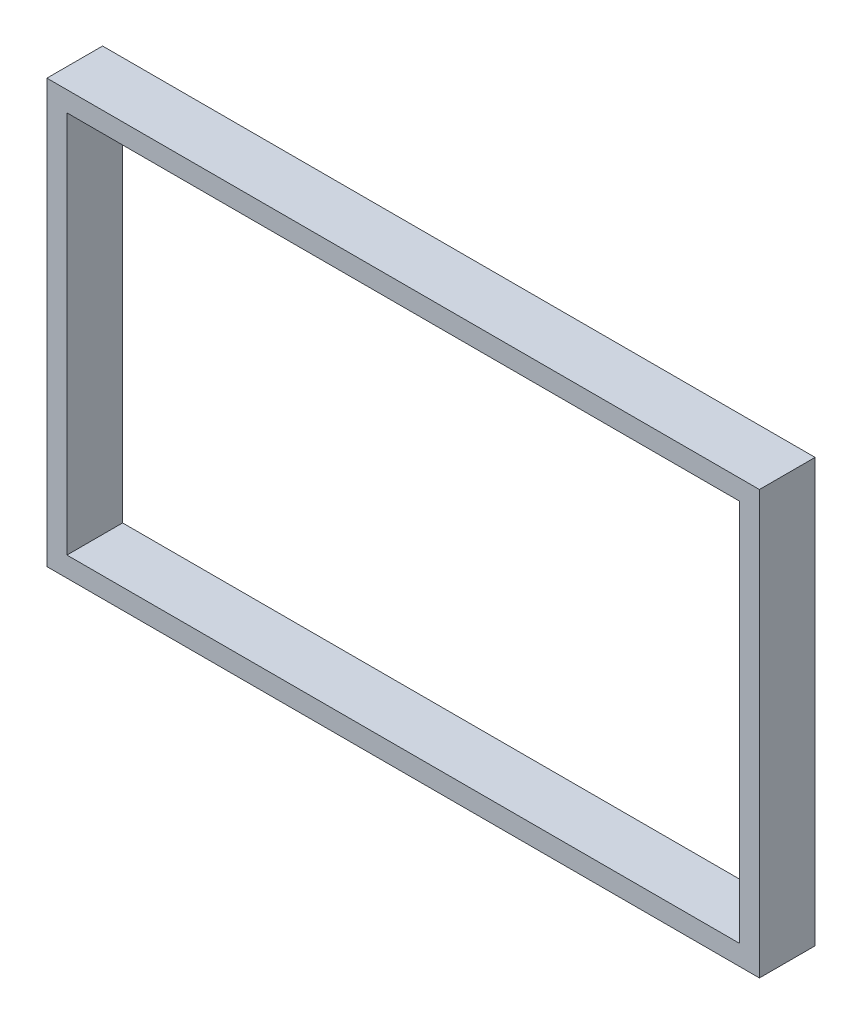
from build123d import *

# Parameters (mm, degrees)
SKETCH_1_W      = 64
SKETCH_1_H      = 38
SKETCH_1_W_2    = 60.4
SKETCH_1_H_2    = 34.4
EXTRUDE_1_DEPTH = 2.5


with BuildPart() as part:
    # 草图1 → 凸台-拉伸1 (new, symmetric)
    with BuildSketch(Plane.XY):
        Rectangle(SKETCH_1_W, SKETCH_1_H)
        Rectangle(SKETCH_1_W_2, SKETCH_1_H_2, mode=Mode.SUBTRACT)
    extrude(amount=EXTRUDE_1_DEPTH, both=True)


solid = part.part
